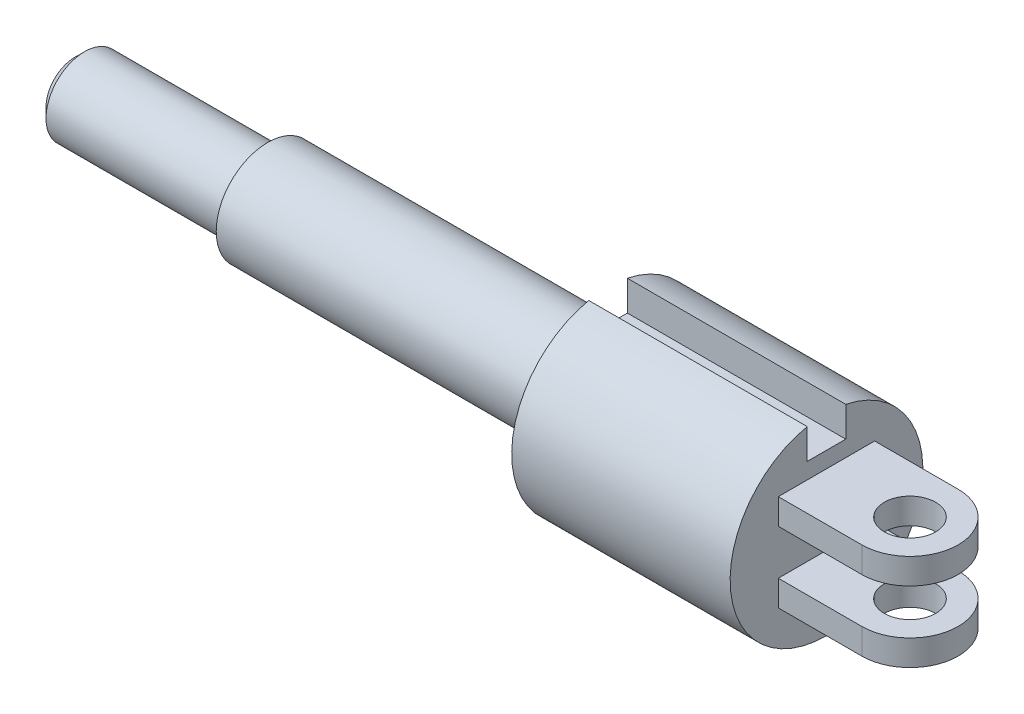
SolidWorks part; units mm, degrees
material "A3"
ref_plane "前视基准面" through (0, 0, 0) normal (0, 0, 1) x (1, 0, 0)
ref_plane "上视基准面" through (0, 0, 0) normal (0, 1, 0) x (1, 0, 0)
ref_plane "右视基准面" through (0, 0, 0) normal (1, 0, 0) x (0, 0, -1)
sketch "草图1" plane through (0, 0, 0) normal (0, 0, 1) x (1, 0, 0)
  line L1 (17, -15) -> (-17, -15)
  line L2 (17, -15) -> (17, 15)
  line L3 (17, 15) -> (-17, 15)
  line L4 (-17, -15) -> (-17, 15)
  line L5 (17, -15) -> (-17, 15) construction
  line L6 (17, 15) -> (-17, -15) construction
  point P0 (0, 0)
  dimension "D1" = 30
  dimension "D2" = 34
extrude "凸台-拉伸1" add sketch "草图1" along normal mid plane 30
sketch "草图6" plane through (17, 0, 0) normal (1, 0, 0) x (0, 0, -1)
  circle A0 centre (0, 0) radius 15
  circle A1 centre (0, 0) radius 25
  dimension "D1" = 30
  dimension "D2" = 50
extrude "切除-拉伸2" cut sketch "草图6" against normal up to surface (34 mm away) up to face at (-17, 0, 0)
sketch "草图2" plane through (0, 0, 0) normal (0, 1, 0) x (1, 0, 0)
  line L1 (-17, -3) -> (17, -3)
  line L2 (-17, -3) -> (-17, 3)
  line L3 (-17, 3) -> (17, 3)
  line L4 (17, -3) -> (17, 3)
  line L5 (-17, -3) -> (17, 3) construction
  line L6 (-17, 3) -> (17, -3) construction
  line L7 (17, -15) -> (17, 15) construction
  point P0 (0, 0)
  dimension "D1" = 6
extrude "切除-拉伸1" cut sketch "草图2" along normal through all from offset 10
sketch "草图3" plane through (-17, 0, 0) normal (-1, 0, 0) x (0, 0, 1)
  circle A0 centre (0, 0) radius 8
  dimension "D1" = 16
extrude "凸台-拉伸2" add sketch "草图3" along normal blind 53
sketch "草图4" plane through (-70, 0, 0) normal (-1, 0, 0) x (0, 0, 1)
  circle A0 centre (0, 0) radius 6
  dimension "D1" = 12
extrude "凸台-拉伸3" add sketch "草图4" along normal blind 30
cosmetic thread "装饰螺纹线1" parameters "D2"=10.106
chamfer "倒角1" distance 1.5 angle 45 1 edges at (-100, 0, 6)
sketch "草图5" plane through (0, 0, 0) normal (0, 1, 0) x (1, 0, 0)
  line L1 (30, -7.5) -> (17, -7.5)
  line L2 (30, -7.5) -> (30, 7.5) construction
  line L3 (30, 7.5) -> (17, 7.5)
  line L4 (17, -7.5) -> (17, 7.5)
  line L5 (30, -7.5) -> (17, 7.5) construction
  line L6 (30, 7.5) -> (17, -7.5) construction
  line L7 (17, -15) -> (17, 15) construction
  arc A1 (30, -7.5) -> (30, 7.5) centre (30, 0) ccw
  circle A2 centre (30, 0) radius 4
  point P0 (23.5, 0)
  dimension "D3" = 8
  dimension "D1" = 13
  dimension "D2" = 15
extrude "凸台-拉伸4" add sketch "草图5" along normal blind 4 from offset 3.5
mirror "镜向1" about plane through (0, 0, 0) normal (0, 1, 0) of "凸台-拉伸4"
